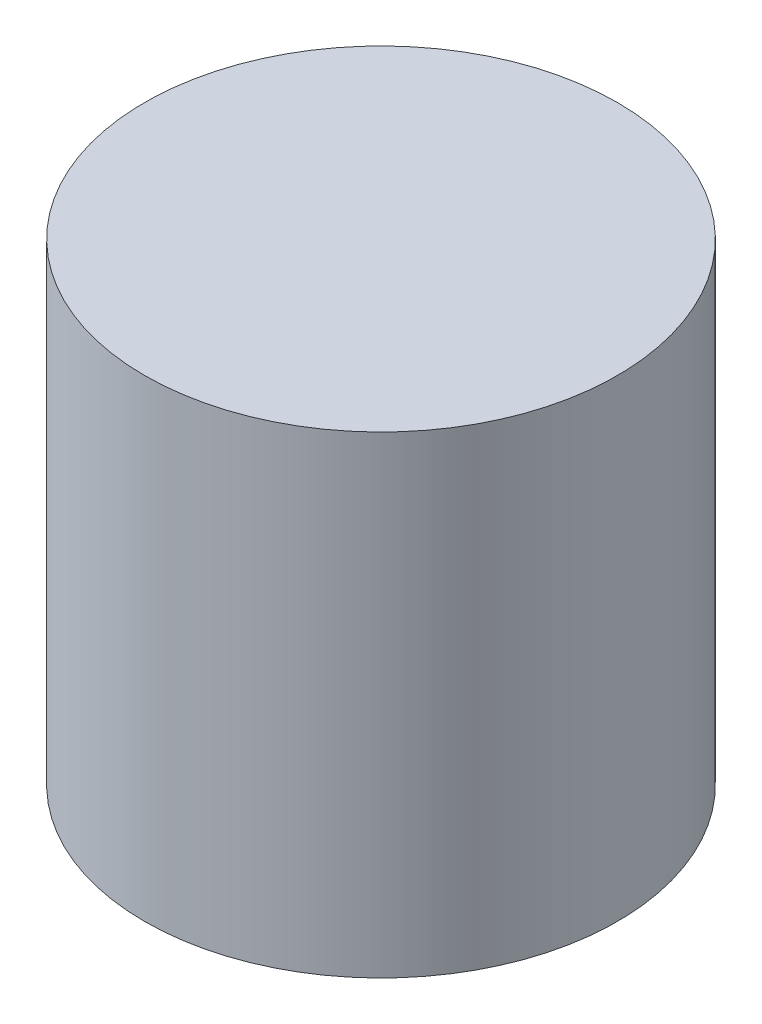
SolidWorks part; units mm, degrees
ref_plane "Front Plane" through (0, 0, 0) normal (0, 0, 1) x (1, 0, 0)
ref_plane "Top Plane" through (0, 0, 0) normal (0, 1, 0) x (1, 0, 0)
ref_plane "Right Plane" through (0, 0, 0) normal (1, 0, 0) x (0, 0, -1)
sketch "Sketch1" plane through (0, 0, 0) normal (0, 0, 1) x (1, 0, 0)
  line L0 (0, 8.6229) -> (0, -3.008) construction
  line L1 (0, 24.4473) -> (10, 24.4473)
  line L2 (10, 24.4473) -> (10, 4.4473)
  line L3 (10, 4.4473) -> (2.5, 4.4473)
  line L4 (2.5, 4.4473) -> (2.5, 0.4473)
  line L5 (2.5, 0.4473) -> (0, 0.4473)
  line L6 (0, 0.4473) -> (0, 24.4473)
  dimension "D1" = 2.5
  dimension "D2" = 10
  dimension "D3" = 20
  dimension "D4" = 4
revolve "Revolve1" add sketch "Sketch1" angle 360 about L0
